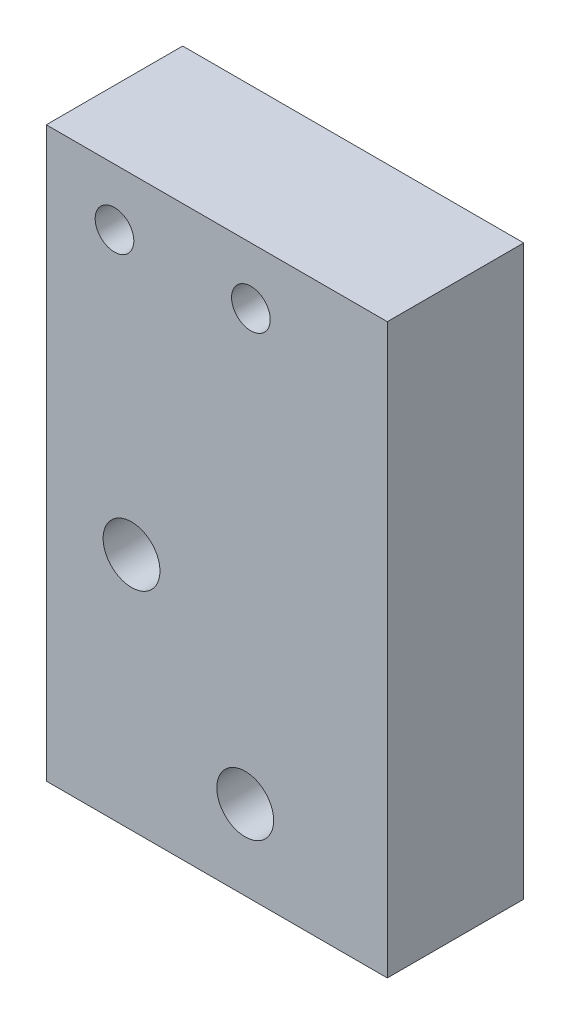
SolidWorks part; units mm, degrees
ref_plane "Front Plane" through (0, 0, 0) normal (0, 0, 1) x (1, 0, 0)
ref_plane "Top Plane" through (0, 0, 0) normal (0, 1, 0) x (1, 0, 0)
ref_plane "Right Plane" through (0, 0, 0) normal (1, 0, 0) x (0, 0, -1)
sketch "Sketch 1" plane through (0, 0, 0) normal (0, 0, 1) x (1, 0, 0)
  line L1 (-15, -25) -> (15, -25)
  line L2 (-15, -25) -> (-15, 25)
  line L3 (-15, 25) -> (15, 25)
  line L4 (15, -25) -> (15, 25)
  line L5 (-15, -25) -> (15, 25) construction
  line L6 (-15, 25) -> (15, -25) construction
  point P0 (0, 0)
  dimension "D1" = 50
  dimension "D2" = 30
extrude "Boss-Extrude 1" add sketch "Sketch 1" along normal blind 12
hole_wizard "M6 Tapped Hole 1" positions "Sketch 3" profile "Sketch 2" tap size "M6" standard "GB" end condition through all
sketch "Sketch 3" plane through (0, 0, 0) normal (0, 0, -1) x (-1, 0, 0)
  line L0 (15, -25) -> (-15, -25) construction
  line L1 (15, 25) -> (15, -25) construction
  point P0 (7.5, -4)
  point P6 (-2.5, -18)
  dimension "D1" = 21
  dimension "D2" = 7.5
  dimension "D3" = 10
  dimension "D4" = 14
sketch "Sketch 2" plane through (-7.5, -4, 0) normal (1, 0, 0) x (0, 1, 0)
  line L0 (0, 0) -> (0, 12)
  line L1 (0, 12) -> (2.5, 12)
  line L2 (2.5, 12) -> (2.5, 0)
  line L5 (2.5, 0) -> (0, 0)
  line L11 (0, -6.35) -> (0, 107.95) construction
  dimension "貫穿螺孔鑽直徑" = 5
  dimension "貫穿螺孔鑽深度" = 12
cosmetic thread "Cosmetic Thread 1"
cosmetic thread "Cosmetic Thread 2"
hole_wizard "M3 Socket Head Cap Screw Counterbore 1" positions "Sketch 5" profile "Sketch 4" counterbore size "M3" standard "JIS" end condition through all
sketch "Sketch 5" plane through (0, 0, 0) normal (0, 0, -1) x (-1, 0, 0)
  line L0 (-15, 25) -> (15, 25) construction
  line L1 (15, 25) -> (15, -25) construction
  point P0 (9, 20)
  dimension "D1" = 5
  dimension "D2" = 6
sketch "Sketch 4" plane through (-9, 20, 0) normal (1, 0, 0) x (0, 1, 0)
  line L0 (0, 0) -> (0, 12)
  line L1 (0, 12) -> (1.7, 12)
  line L3 (1.7, 12) -> (1.7, 3)
  line L4 (1.7, 3) -> (3.25, 3)
  line L5 (3.25, 3) -> (3.25, 0)
  line L7 (3.25, 0) -> (0, 0)
  line L11 (0, -6.35) -> (0, 107.95) construction
  dimension "貫穿孔直徑" = 3.4
  dimension "貫穿孔深度" = 12
  dimension "柱孔直徑" = 6.5
  dimension "柱孔深度" = 3
pattern_linear "Linear Pattern 1" count 2 spacing 12 along (1, 0, 0) of "M3 Socket Head Cap Screw Counterbore 1"
